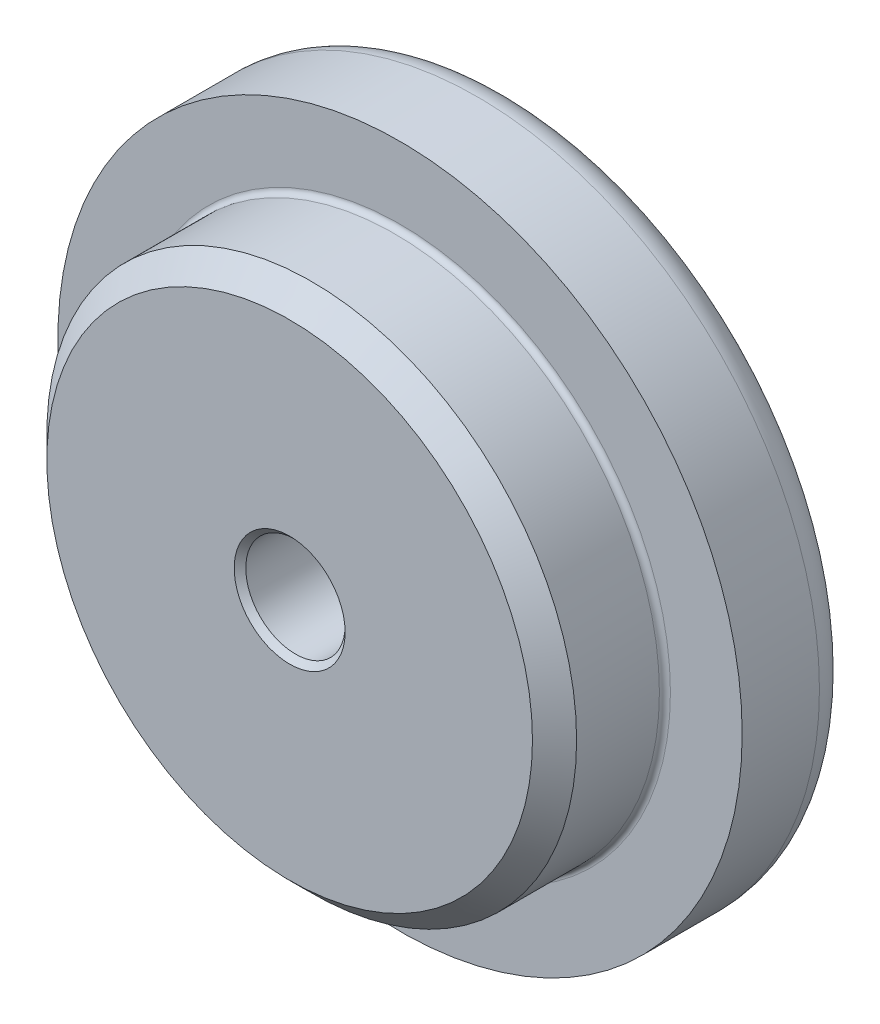
from build123d import *

# Parameters (mm, degrees)
SKETCH_1_R            = 31
EXTRUDE_1_DEPTH       = 10
SKETCH_2_R            = 24
EXTRUDE_2_DEPTH       = 10
CHAMFER_1_SIZE        = 2
FILLET_1_R            = 3
M10X1_0_1_D           = 9
M10X1_0_1_DEPTH       = 25
M10X1_0_1_CSINK_D     = 10.05
M10X1_0_1_CSINK_ANGLE = 90
M10X1_0_1_TIP         = 2.703872786
CUT_EXTRUDE_1_DEPTH   = 1
CUT_EXTRUDE_2_DEPTH   = 1
FILLET_2_R            = 0.5


with BuildPart() as part:
    # 草图1 → 凸台-拉伸1 (new body)
    with BuildSketch(Plane.XY):
        Circle(SKETCH_1_R)
    extrude(amount=EXTRUDE_1_DEPTH)

    # 草图2 → 凸台-拉伸2 (add)
    with BuildSketch(Plane.XY.offset(10)):
        Circle(SKETCH_2_R)
    extrude(amount=EXTRUDE_2_DEPTH)

    # 倒角1
    chamfer_1_edges = [part.edges().sort_by_distance(p)[0] for p in [
        (-24, 0, 20),
    ]]
    chamfer(chamfer_1_edges, length=CHAMFER_1_SIZE)

    # 圆角1
    fillet_1_edges = [part.edges().sort_by_distance(p)[0] for p in [
        (-31, 0, 0),
    ]]
    fillet(fillet_1_edges, radius=FILLET_1_R)

    # M10x1.0 螺纹孔1
    with Locations(Plane.XY.offset(20)):
        with Locations((0, 0)):
            CounterSinkHole(M10X1_0_1_D / 2, M10X1_0_1_CSINK_D / 2, depth=M10X1_0_1_DEPTH, counter_sink_angle=M10X1_0_1_CSINK_ANGLE)
            with Locations((0, 0, -(M10X1_0_1_DEPTH + M10X1_0_1_TIP / 2))):  # 118° drill point
                Cone(0, M10X1_0_1_D / 2, M10X1_0_1_TIP, mode=Mode.SUBTRACT)

    # 草图4 → 切除-拉伸1 (cut)
    with BuildSketch(Plane(origin=(0, 0, 0), x_dir=(-1, 0, 0), z_dir=(0, 0, -1))):
        with BuildLine():
            Line((-3, -25), (-3, 25))
            ThreePointArc((-3, 25), (0, 28), (3, 25))
            Line((3, 25), (3, -25))
            ThreePointArc((3, -25), (0, -28), (-3, -25))
        make_face()
    extrude(amount=-CUT_EXTRUDE_1_DEPTH, mode=Mode.SUBTRACT)

    # 草图5 → 切除-拉伸2 (cut)
    with BuildSketch(Plane(origin=(0, 0, 0), x_dir=(-1, 0, 0), z_dir=(0, 0, -1))):
        with BuildLine():
            Line((-25, 3), (25, 3))
            ThreePointArc((25, 3), (28, 0), (25, -3))
            Line((25, -3), (-25, -3))
            ThreePointArc((-25, -3), (-28, 0), (-25, 3))
        make_face()
    extrude(amount=-CUT_EXTRUDE_2_DEPTH, mode=Mode.SUBTRACT)

    # 圆角2
    fillet_2_edges = [part.edges().sort_by_distance(p)[0] for p in [
        (-24, 0, 10),
    ]]
    fillet(fillet_2_edges, radius=FILLET_2_R)


solid = part.part
